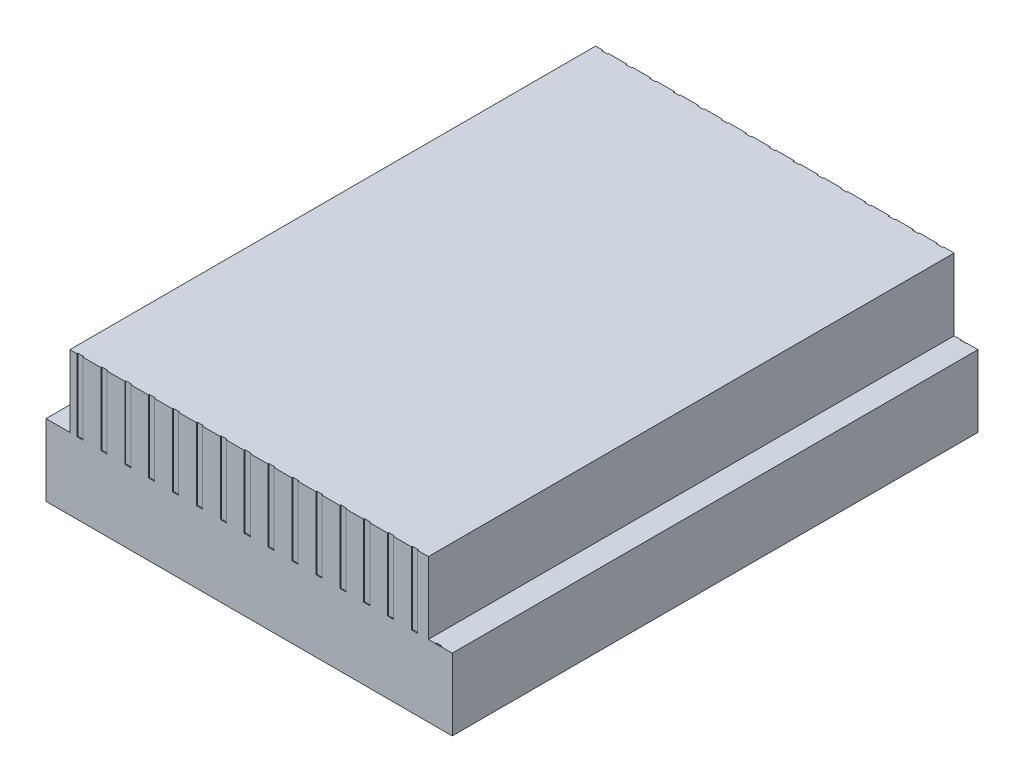
SolidWorks part; units mm, degrees
ref_plane "Front Plane" through (0, 0, 0) normal (0, 0, 1) x (1, 0, 0)
ref_plane "Top Plane" through (0, 0, 0) normal (0, 1, 0) x (1, 0, 0)
ref_plane "Right Plane" through (0, 0, 0) normal (1, 0, 0) x (0, 0, -1)
other "Configuration Table"
sketch "Sketch1" plane through (0, 0, 0) normal (0, 0, 1) x (1, 0, 0)
  line L0 (0, 0) -> (100, 0)
  line L1 (0, 0) -> (0, 120)
  line L2 (15, 15) -> (20, 15)
  line L3 (15, 15) -> (15, 120)
  line L4 (15, 120) -> (0, 120)
  line L5 (100, 15) -> (100, 0)
  line L6 (20, 15) -> (20, 30)
  line L7 (20, 30) -> (95, 30)
  line L8 (95, 30) -> (95, 15)
  line L9 (95, 15) -> (100, 15)
  line L10 (15, 15) -> (100, 15) construction
  dimension "D1" = 100
  dimension "D2" = 120
  dimension "D4" = 15
  dimension "D5" = 5
  dimension "D6" = 5
  dimension "D3" = 15
extrude "Boss-Extrude1" add sketch "Sketch1" along normal blind 110
sketch "Sketch2" plane through (0, 0, 110) normal (0, 0, 1) x (1, 0, 0)
  line L0 (95, 30) -> (20, 30) construction
  line L1 (21.4792, 30) -> (22.7391, 30)
  line L2 (21.4792, 30) -> (21.4792, 14.9569)
  line L3 (21.4792, 14.9569) -> (22.7391, 14.9569)
  line L4 (22.7391, 30) -> (22.7391, 14.9569)
  line L5 (21.4792, 30) -> (22.7391, 14.9569) construction
  line L6 (21.4792, 14.9569) -> (22.7391, 30) construction
  point P0 (22.1092, 22.4785)
extrude "Cut-Extrude1" cut sketch "Sketch2" against normal blind 0.2
pattern_linear "LPattern1" count 16 spacing 5 along (1, 0, 0) of "Cut-Extrude1"
ref_plane "Plane1" through (0, 0, 55) normal (0, 0, -1) x (-1, 0, 0)
mirror "Mirror1" about plane through (0, 0, 55) normal (0, 0, -1) of "LPattern1", "Cut-Extrude1"
sketch "Sketch4" plane through (0, 0, 0) normal (0, 0, -1) x (-1, 0, 0)
  line L1 (-15, 120) -> (23.9587, 120)
  line L2 (-15, 120) -> (-15, -17.4014)
  line L3 (-15, -17.4014) -> (23.9587, -17.4014)
  line L4 (23.9587, 120) -> (23.9587, -17.4014)
extrude "Cut-Extrude2" cut sketch "Sketch4" against normal through all
